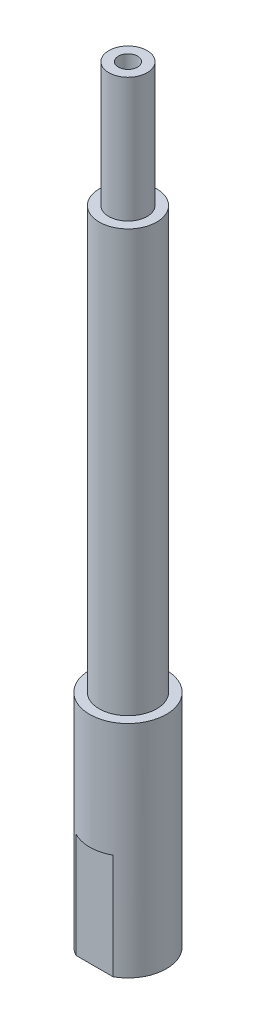
from build123d import *

# Parameters (mm, degrees)
SKETCH5_R                  = 1
CUT_EXTRUDE2_DEPTH         = 81.199750623
M5X0_75_TAPPED_HOLE1_D     = 4.2
M5X0_75_TAPPED_HOLE1_DEPTH = 12.25
M5X0_75_TAPPED_HOLE1_TIP   = 1.2618073
CUT_EXTRUDE3_DEPTH         = 81.199750623
CUT_EXTRUDE3_DEPTH_BACK    = 81.199750623
SKETCH6_W                  = 4.168944331
SKETCH6_H                  = 22.175025747
SKETCH6_W_2                = 2.42822795
SKETCH7_R                  = 3
BOSS_EXTRUDE1_DEPTH        = 5


with BuildPart() as part:
    # Sketch1 → Revolve1 (revolve)
    with BuildSketch(Plane.XY, mode=Mode.PRIVATE) as revolve1_sk:
        Polygon((3, 23), (4, 23), (4, 0), (0, 0), (0, 80), (2, 80), (2, 62), (3, 62), align=None)
    revolve(revolve1_sk.sketch.rotate(Axis((0, 80, 0), (0, -1, 0)), 180), axis=Axis((0, 80, 0), (0, -1, 0)))

    # Sketch5 → Cut-Extrude2 (cut, through all)
    with BuildSketch(Plane(origin=(0, 80, 0), x_dir=(1, 0, 0), z_dir=(0, 1, 0))):
        with Locations(Location((0, 0, 0), (0, 0, 180))):
            Circle(SKETCH5_R)
    extrude(amount=-CUT_EXTRUDE2_DEPTH, mode=Mode.SUBTRACT)

    # M5x0.75 Tapped Hole1
    with Locations(Plane(origin=(0, 0, 0), x_dir=(-1, 0, 0), z_dir=(0, -1, 0))):
        with Locations((0, 0)):
            Hole(M5X0_75_TAPPED_HOLE1_D / 2, depth=M5X0_75_TAPPED_HOLE1_DEPTH)
            with Locations((0, 0, -(M5X0_75_TAPPED_HOLE1_DEPTH + M5X0_75_TAPPED_HOLE1_TIP / 2))):  # 118° drill point
                Cone(0, M5X0_75_TAPPED_HOLE1_D / 2, M5X0_75_TAPPED_HOLE1_TIP, mode=Mode.SUBTRACT)

    # Sketch6 → Cut-Extrude3 (cut, two sides: drawn at the far end of the back side and taken through both)
    with BuildSketch(Plane(origin=(0, 0, 0), x_dir=(0, 0, -1), z_dir=(1, 0, 0)).offset(-CUT_EXTRUDE3_DEPTH_BACK)):
        with Locations((-5.584472166, -0.087512874)):
            Rectangle(SKETCH6_W, SKETCH6_H)
        with Locations((4.714113975, -0.087512874)):
            Rectangle(SKETCH6_W_2, SKETCH6_H)
    extrude(amount=CUT_EXTRUDE3_DEPTH + CUT_EXTRUDE3_DEPTH_BACK, mode=Mode.SUBTRACT)

    # Sketch7 → Boss-Extrude1 (add)
    with BuildSketch(Plane(origin=(0, 62, 0), x_dir=(1, 0, 0), z_dir=(0, 1, 0))):
        with Locations(Location((0, 0, 0), (0, 0, 180))):
            Circle(SKETCH7_R)
    extrude(amount=BOSS_EXTRUDE1_DEPTH)


solid = part.part
